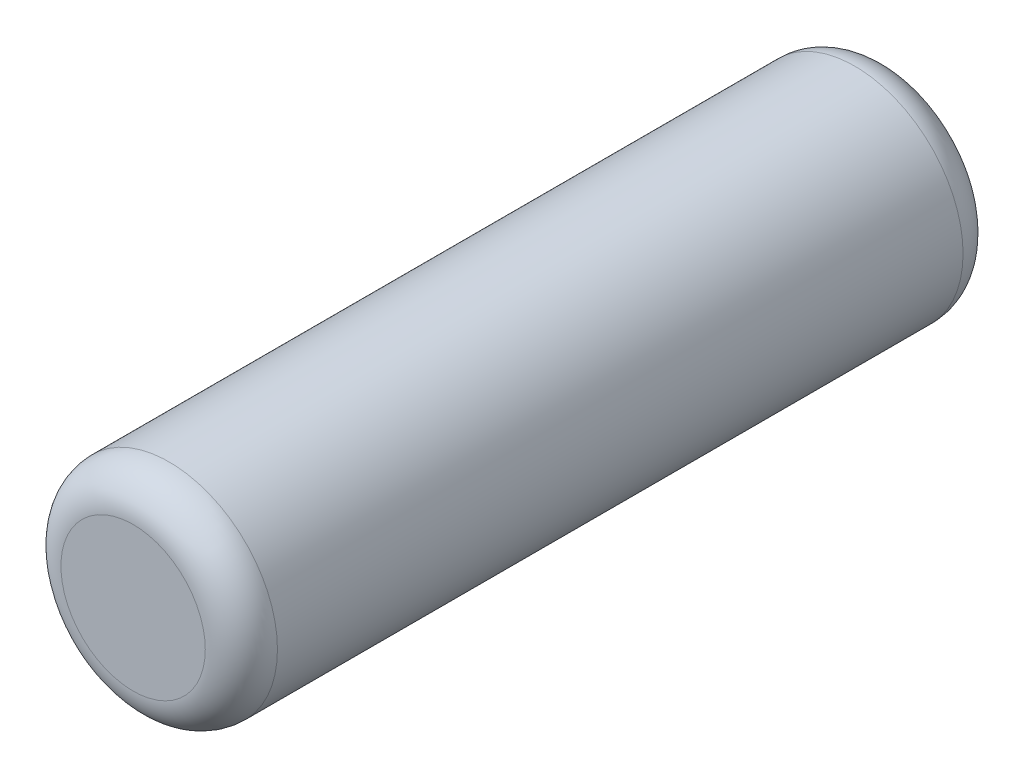
from build123d import *

# Parameters (mm, degrees)
SKETCH1_R           = 3
BOSS_EXTRUDE1_DEPTH = 21
FILLET1_R           = 1


with BuildPart() as part:
    # Sketch1 → Boss-Extrude1 (new body)
    with BuildSketch(Plane.XY):
        with Locations(Location((0, 0, 0), (0, 0, 180))):
            Circle(SKETCH1_R)
    extrude(amount=BOSS_EXTRUDE1_DEPTH)

    # Fillet1
    fillet1_edges = [part.edges().sort_by_distance(p)[0] for p in [
        (3, 0, 0),
        (3, 0, 21),
    ]]
    fillet(fillet1_edges, radius=FILLET1_R)


solid = part.part
